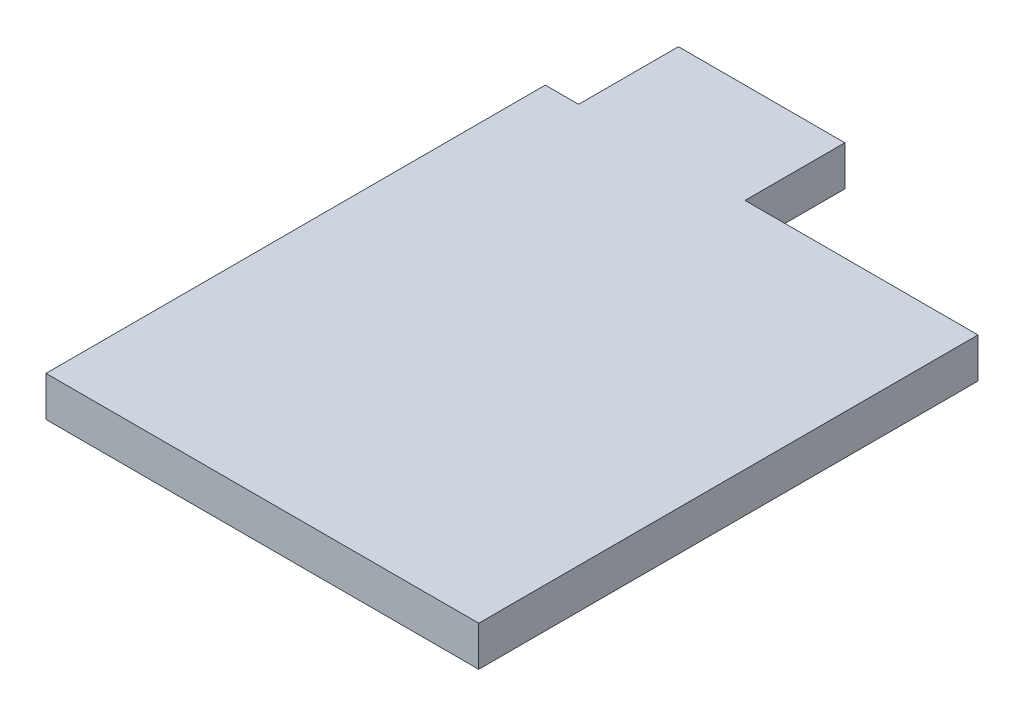
from build123d import *

# Parameters (mm, degrees)
EXTRUDE_1_DEPTH = 12


with BuildPart() as part:
    # 草图1 → 凸台-拉伸1 (new body)
    with BuildSketch(Plane(origin=(0, 0, 0), x_dir=(1, 0, 0), z_dir=(0, 1, 0))):
        Polygon((0, 0), (130, 0), (130, 150), (60, 150), (60, 180), (10, 180), (10, 150), (0, 150), align=None)
    extrude(amount=EXTRUDE_1_DEPTH)


solid = part.part
